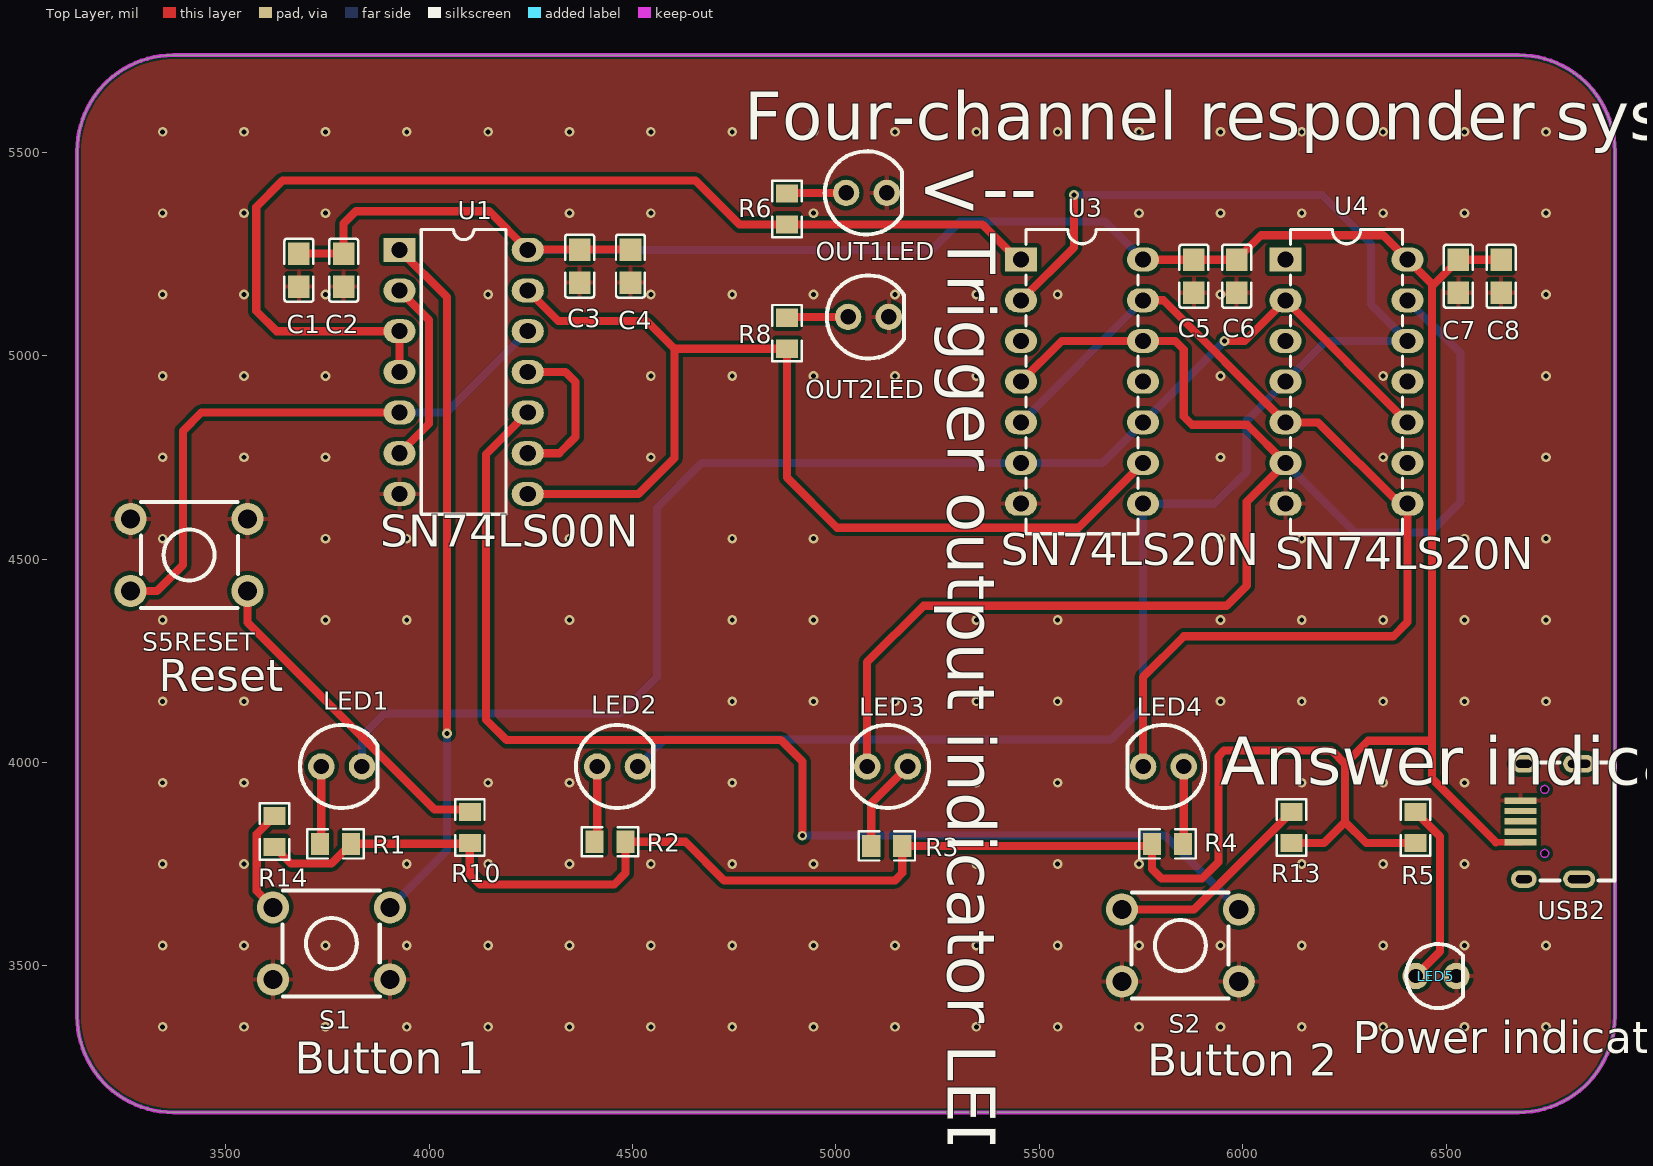
[diagram p0: Top Layer view]
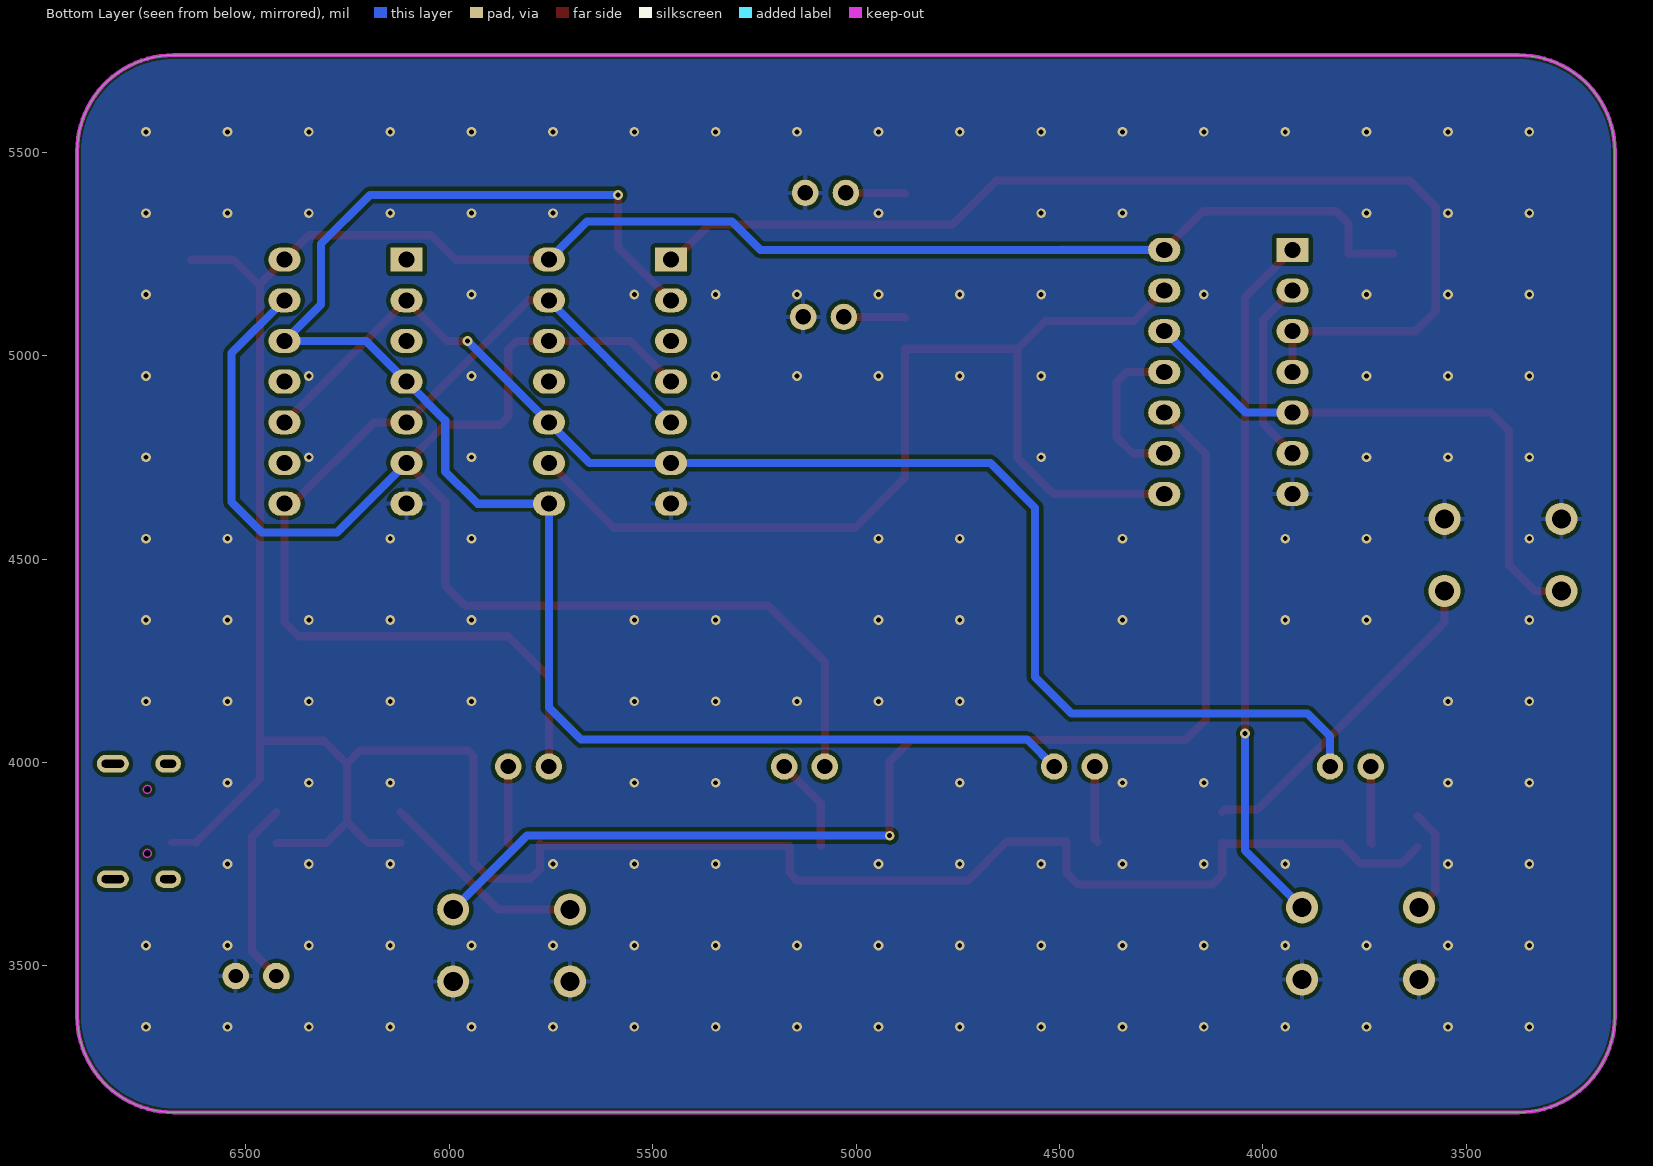
[diagram p1: Bottom Layer view, seen from below]
# Altium PCB MISC75096.pcbdoc
Units mil, origin at the board's own origin, x right, y up, seen from the top; angles counter-clockwise.
Board outline 3779.53 x 2598.43 mil, 2 copper layers (Top Layer, Bottom Layer), stack 62.206 mil thick; 32 components, 29 nets, 113 pads, 159 vias.

## Layer stack, top to bottom
Top Solder Mask Layer: solder mask 0.394, Dk 3.3
Top Layer: signal copper 1.379
Dielectric1: surface 59.449, FR4, Dk 4.5
Bottom Layer: signal copper 1.378
Bottom Solder Mask Layer: solder mask 0.394, Dk 3.3

## Board outline
3135,5502.2 cw(c3371.22,5502.2) 3371.22,5738.43 6678.31,5738.43 cw(c6678.31,5502.2) 6914.53,5502.2 6914.53,3376.22 cw(c6678.31,3376.22) 6678.31,3140 3371.22,3140 cw(c3371.22,3376.22) 3135,3376.22

## Design rules (kind name [scope] priority, off if disabled: settings)
BoardOutlineClearance Plane_innerPlane_1 [All] p2 off: genericclearance=6 ignorepadtopadclearanceinfootprint=FALSE except(0: Arc-SplitContinuation Track-SplitContinuation SMDPad-SplitContinuation THPad-SplitContinuation Via-SplitContinuation Fill-SplitContinuation Region-SplitContinuation Poly-SplitContinuation Text-SplitContinuation Hole-SplitContinuation; 6: Arc-CutoutEdge Track-CutoutEdge SMDPad-CutoutEdge THPad-CutoutEdge Via-CutoutEdge Fill-CutoutEdge Region-CutoutEdge Text-CutoutEdge; 6.9: Hole-OutlineEdge Hole-CutoutEdge; 10: Poly-OutlineEdge Poly-CutoutEdge; 11.8: Arc-OutlineEdge Track-OutlineEdge SMDPad-OutlineEdge THPad-OutlineEdge Via-OutlineEdge Fill-OutlineEdge Region-OutlineEdge Text-OutlineEdge)
BoardOutlineClearance Copper_copperRegion_1 [All] p4 off: genericclearance=6 ignorepadtopadclearanceinfootprint=FALSE except(0: Arc-SplitContinuation Track-SplitContinuation SMDPad-SplitContinuation THPad-SplitContinuation Via-SplitContinuation Fill-SplitContinuation Region-SplitContinuation Poly-SplitContinuation Text-SplitContinuation Hole-SplitContinuation; 6: Arc-CutoutEdge Track-CutoutEdge SMDPad-CutoutEdge THPad-CutoutEdge Via-CutoutEdge Fill-CutoutEdge Region-CutoutEdge Text-CutoutEdge; 6.9: Hole-OutlineEdge Hole-CutoutEdge; 10: Poly-OutlineEdge Poly-CutoutEdge; 11.8: Arc-OutlineEdge Track-OutlineEdge SMDPad-OutlineEdge THPad-OutlineEdge Via-OutlineEdge Fill-OutlineEdge Region-OutlineEdge Text-OutlineEdge)
BoardOutlineClearance Copper_gge8956_1 [All] p6 off: genericclearance=6 ignorepadtopadclearanceinfootprint=FALSE except(0: Arc-SplitContinuation Track-SplitContinuation SMDPad-SplitContinuation THPad-SplitContinuation Via-SplitContinuation Fill-SplitContinuation Region-SplitContinuation Poly-SplitContinuation Text-SplitContinuation Hole-SplitContinuation; 6: Arc-CutoutEdge Track-CutoutEdge SMDPad-CutoutEdge THPad-CutoutEdge Via-CutoutEdge Fill-CutoutEdge Region-CutoutEdge Text-CutoutEdge; 6.9: Hole-OutlineEdge Hole-CutoutEdge; 10: Poly-OutlineEdge Poly-CutoutEdge; 11.8: Arc-OutlineEdge Track-OutlineEdge SMDPad-OutlineEdge THPad-OutlineEdge Via-OutlineEdge Fill-OutlineEdge Region-OutlineEdge Text-OutlineEdge)
BoardOutlineClearance Copper_gge8950_1 [All] p8 off: genericclearance=6 ignorepadtopadclearanceinfootprint=FALSE except(0: Arc-SplitContinuation Track-SplitContinuation SMDPad-SplitContinuation THPad-SplitContinuation Via-SplitContinuation Fill-SplitContinuation Region-SplitContinuation Poly-SplitContinuation Text-SplitContinuation Hole-SplitContinuation; 6: Arc-CutoutEdge Track-CutoutEdge SMDPad-CutoutEdge THPad-CutoutEdge Via-CutoutEdge Fill-CutoutEdge Region-CutoutEdge Text-CutoutEdge; 6.9: Hole-OutlineEdge Hole-CutoutEdge; 10: Poly-OutlineEdge Poly-CutoutEdge; 11.8: Arc-OutlineEdge Track-OutlineEdge SMDPad-OutlineEdge THPad-OutlineEdge Via-OutlineEdge Fill-OutlineEdge Region-OutlineEdge Text-OutlineEdge)
BoardOutlineClearance safeClearance_1 [All] p10: genericclearance=6 ignorepadtopadclearanceinfootprint=FALSE except(0: Arc-SplitContinuation Track-SplitContinuation SMDPad-SplitContinuation THPad-SplitContinuation Via-SplitContinuation Fill-SplitContinuation Region-SplitContinuation Poly-SplitContinuation Text-SplitContinuation Hole-SplitContinuation; 6: Arc-CutoutEdge Track-CutoutEdge SMDPad-CutoutEdge THPad-CutoutEdge Via-CutoutEdge Fill-CutoutEdge Region-CutoutEdge Text-CutoutEdge; 6.9: Hole-OutlineEdge Hole-CutoutEdge; 10: Poly-OutlineEdge Poly-CutoutEdge; 11.8: Arc-OutlineEdge Track-OutlineEdge SMDPad-OutlineEdge THPad-OutlineEdge Via-OutlineEdge Fill-OutlineEdge Region-OutlineEdge Text-OutlineEdge)
Clearance Plane_innerPlane [All] p1 off: gap=6 ignorepadtopadclearanceinfootprint=FALSE except(6.9: Hole-Track Hole-SMDPad Hole-THPad Hole-Via Fill-Hole Region-Hole Hole-Arc Hole-Text; 10: Poly-Track Poly-SMDPad Poly-THPad Poly-Via Poly-Fill Poly-Region Poly-Poly Poly-Arc Poly-Text Poly-Hole)
Clearance Copper_copperRegion [All] p3 off: gap=6 ignorepadtopadclearanceinfootprint=FALSE except(6.9: Hole-Track Hole-SMDPad Hole-THPad Hole-Via Fill-Hole Region-Hole Hole-Arc Hole-Text; 10: Poly-Track Poly-SMDPad Poly-THPad Poly-Via Poly-Fill Poly-Region Poly-Poly Poly-Arc Poly-Text Poly-Hole)
Clearance Copper_gge8956 [All] p5 off: gap=6 ignorepadtopadclearanceinfootprint=FALSE except(6.9: Hole-Track Hole-SMDPad Hole-THPad Hole-Via Fill-Hole Region-Hole Hole-Arc Hole-Text; 10: Poly-Track Poly-SMDPad Poly-THPad Poly-Via Poly-Fill Poly-Region Poly-Poly Poly-Arc Poly-Text Poly-Hole)
Clearance Copper_gge8950 [All] p7 off: gap=6 ignorepadtopadclearanceinfootprint=FALSE except(6.9: Hole-Track Hole-SMDPad Hole-THPad Hole-Via Fill-Hole Region-Hole Hole-Arc Hole-Text; 10: Poly-Track Poly-SMDPad Poly-THPad Poly-Via Poly-Fill Poly-Region Poly-Poly Poly-Arc Poly-Text Poly-Hole)
Clearance safeClearance [All] p9: gap=6 ignorepadtopadclearanceinfootprint=FALSE except(6.9: Hole-Track Hole-SMDPad Hole-THPad Hole-Via Fill-Hole Region-Hole Hole-Arc Hole-Text; 10: Poly-Track Poly-SMDPad Poly-THPad Poly-Via Poly-Fill Poly-Region Poly-Poly Poly-Arc Poly-Text Poly-Hole)
DiffPairsRouting differentialPair [All] p1: maxlimit=6 minlimit=6 mostfreqgap=6 toplayer_minwidth=5 toplayer_prefwidth=10 toplayer_maxwidth=100 toplayer_mingap=6 toplayer_prefgap=6 toplayer_maxgap=6 bottomlayer_minwidth=5 bottomlayer_prefwidth=10 bottomlayer_maxwidth=100 bottomlayer_mingap=6 bottomlayer_prefgap=6 bottomlayer_maxgap=6 maxuncoupledlength=10
HoleToHoleClearance gge8956 [All] p1 off: gap=0 allowstackedmicrovias=TRUE
HoleToHoleClearance gge8950 [All] p2 off: gap=0 allowstackedmicrovias=TRUE
HoleToHoleClearance Common [All] p3: gap=11.8 allowstackedmicrovias=TRUE
Length netLength [All] p1: minlimit=0 maxlimit=0
PasteMaskExpansion pasteMaskExpansion [All] p1: expansion=0
PlaneConnect innerPlane [All] p1: planeconnectstyle=Relief reliefexpansion=20 reliefentries=4 reliefconductorwidth=10 reliefairgap=10
PolygonConnect gge8956_1 [All] p1 off: connectstyle=Relief reliefconductorwidth=10 reliefentries=4 polygonreliefangle="90 Angle" airgapwidth=10 via.connectstyle=Relief via.reliefconductorwidth=10 via.reliefentries=4 via.polygonreliefangle="90 Angle" via.airgapwidth=10
PolygonConnect gge8950_1 [All] p2 off: connectstyle=Relief reliefconductorwidth=10 reliefentries=4 polygonreliefangle="90 Angle" airgapwidth=10 via.connectstyle=Relief via.reliefconductorwidth=10 via.reliefentries=4 via.polygonreliefangle="90 Angle" via.airgapwidth=10
PolygonConnect copperRegion [All] p3: connectstyle=Relief reliefconductorwidth=10 reliefentries=4 polygonreliefangle="90 Angle" airgapwidth=10 via.connectstyle=Relief via.reliefconductorwidth=10 via.reliefentries=4 via.polygonreliefangle="90 Angle" via.airgapwidth=10
RoutingVias viaSize [All] p1: holewidth=12 width=24 viastyle="Through Hole" minholewidth=11.8 minwidth=19.7 maxholewidth=236.2 maxwidth=393.7
SolderMaskExpansion solderMaskExpansion [IsVia] p1: expansion=-1000 istentingtop=TRUE
SolderMaskExpansion solderMaskExpansion [All] p2: expansion=2 istentingtop=FALSE
Width trackWidth [All] p1: maxlimit=100 minlimit=5 preferedwidth=20

## Components (designator, comment, footprint, x,y, rotation, side; value= is the part's Value field where it differs from the comment)
C1 "10u" C0805 3680,5210 r270 top
C2 "0.1u" C0805 3790,5210 r270 top
C3 "10u" C0805 4370,5220 r270 top
C4 "0.1u" C0805 4495,5220 r270 top
C5 "10u" C0805 5880,5195 r270 top
C6 "0.1u" C0805 5985,5195 r270 top
C7 "10u" C0805 6530,5195 r270 top
C8 "0.1u" C0805 6635,5195 r270 top
LED1 "LED-TH-5mm_R" LED-TH_BD5.0_RED 3785,3989.99 r90 top
LED2 "LED-TH-5mm_R" LED-TH_BD5.0_RED 4463.2,3989.99 r90 top
LED3 "LED-TH-5mm_R" LED-TH_BD5.0_RED 5126.8,3990 r270 top
LED4 "LED-TH-5mm_R" LED-TH_BD5.0_RED 5805,3990 r270 top
LED5 "LED-TH-3mm_R" LED-TH_BD3.0_RED 6475,3475 r90 top
OUT1LED "LED-TH-5mm_R" LED-TH_BD5.0_RED 5075,5400 r90 top
OUT2LED "LED-TH-5mm_R" LED-TH_BD5.0_RED 5080,5095 r90 top
R1 "1k" R0805 3770,3800 r0 top
R2 "1k" R0805 4445,3805 r0 top
R3 "1k" R0805 5125,3795 r0 top
R4 "1k" R0805 5815,3800 r180 top
R5 "1k" R0805 6425,3840 r90 top
R6 "1k" R0805 4880,5360 r90 top
R8 "1k" R0805 4880,5055 r90 top
R10 "1k" R0805 4100,3840 r90 top
R13 "1k" R0805 6120,3840 r90 top
R14 "1k" R0805 3620,3830 r90 top
S1 "TC-1157-B-A" KEY-TH_4P-L6.4-W6.0-P4.50-LS7.3-TL 3760,3555 r0 top
S2 "TC-1157-B-A" KEY-TH_4P-L6.4-W6.0-P4.50-LS7.3-TL 5846.67,3550 r0 top
S5RESET "TC-1157-B-A" KEY-TH_4P-L6.4-W6.0-P4.50-LS7.3-TL 3410,4510 r180 top
U1 "SN74LS00N" PDIP-14_L19.7-W6.6-P2.54-LS8.3-BL 4085,4960 r270 top
U3 "SN74LS20N" DIP-14_L19.0-W7.0-P2.54-LS7.6-BL 5605,4935.98 r270 top
U4 "SN74LS20N" DIP-14_L19.0-W7.0-P2.54-LS7.6-BL 6255,4935.98 r270 top
USB2 "U-F-M5DD-W-2-SUS" MICRO-USB-SMD_U-F-M5DD-W-2-SUS 6755,3855 r270 top

## Footprints (in the part's own frame and the unit in brackets; to place one, negate y for a bottom-side part, rotate by r counter-clockwise, add the part's x,y. Pads: shape width x height; smd on the part's side, far side on the other; paste and mask are expansions set on the pad)
C0805 [mm]
  rect 1.41x1.35 smd paste-100 mask+0.051: 1(-1.03,0) 2(1.03,0)
  silkscreen extent -1.96,-0.9 1.96,0.9
DIP-14_L19.0-W7.0-P2.54-LS7.6-BL [mm]
  rect 1.5x2 hole 1: 1(-7.62,-3.81)
  oval 1.5x2 hole 1: 2(-5.08,-3.81) 3(-2.54,-3.81) 4(0,-3.81) 5(2.54,-3.81) 6(5.08,-3.81) 7(7.62,-3.81) 8(7.62,3.81) 9(5.08,3.81) 10(2.54,3.81) 11(0,3.81) 12(-2.54,3.81) 13(-5.08,3.81) 14(-7.62,3.81)
  silkscreen extent -9.5,-3.5 9.5,3.5
KEY-TH_4P-L6.4-W6.0-P4.50-LS7.3-TL [mm]
  round 2 hole 1.2: 1(-3.65,2.25) 2(3.65,2.25) 3(-3.65,-2.25)
  round 2 hole 1.2 copper offset 0,0: 4(3.65,-2.25)
  silkscreen extent -3.05,-3.3 3.01,3.3
LED-TH_BD3.0_RED [mil]
  round 65 hole 35.43: 1(0,50) 2(0,-50)
  silkscreen extent -79,-66 79,73
LED-TH_BD5.0_RED [mil]
  round 65 hole 38: 1(0,50) 2(0,-50)
  silkscreen extent -102,-88 102,102
MICRO-USB-SMD_U-F-M5DD-W-2-SUS [mm]
  rect 0.4x2 smd paste-100 mask+0.051: 1(1.3,-1.825) 2(0.65,-1.825) 3(0,-1.825) 4(-0.65,-1.825) 5(-1.3,-1.825)
  oval 1.1x1.6 hole 0.5 slot 1 at 90 deg: 6(-3.6,-1.625) 8(3.6,-1.625)
  oval 1.1x2 hole 0.5 slot 1.4 at 90 deg: 7(-3.6,1.825) 9(3.6,1.825)
  Board Outline Layer circle w0.003: c-2,-0.325 r0.25
  Board Outline Layer circle w0.003: c2,-0.325 r0.25
  Board Outline Layer region: -2,-0.075 -1.892,-0.1 -1.805,-0.169 -1.756,-0.269 -1.756,-0.38 -1.805,-0.481 -1.892,-0.55 -2,-0.575 -2,-0.575 -2.108,-0.55 -2.195,-0.481 -2.244,-0.38 -2.244,-0.269 -2.195,-0.169 -2.108,-0.1 -2,-0.075
  Board Outline Layer region: -2,-0.075 -1.935,-0.083 -1.875,-0.108 -1.823,-0.148 -1.783,-0.2 -1.759,-0.26 -1.75,-0.325 -1.759,-0.39 -1.783,-0.45 -1.823,-0.502 -1.875,-0.541 -1.935,-0.566 -2,-0.575 -2.065,-0.566 -2.125,-0.541 -2.177,-0.502 -2.217,-0.45 -2.241,-0.39 -2.25,-0.325 -2.241,-0.26 -2.217,-0.2 -2.177,-0.148 -2.125,-0.108 -2.065,-0.083
  Board Outline Layer region: 2,-0.075 2.108,-0.1 2.195,-0.169 2.244,-0.269 2.244,-0.38 2.195,-0.481 2.108,-0.55 2,-0.575 2,-0.575 1.892,-0.55 1.805,-0.481 1.756,-0.38 1.756,-0.269 1.805,-0.169 1.892,-0.1 2,-0.075
  Board Outline Layer region: 2,-0.075 2.065,-0.083 2.125,-0.108 2.177,-0.148 2.217,-0.2 2.241,-0.26 2.25,-0.325 2.241,-0.39 2.217,-0.45 2.177,-0.502 2.125,-0.541 2.065,-0.566 2,-0.575 1.935,-0.566 1.875,-0.541 1.823,-0.502 1.783,-0.45 1.759,-0.39 1.75,-0.325 1.759,-0.26 1.783,-0.2 1.823,-0.148 1.875,-0.108 1.935,-0.083
  Multi-Layer board cut-out: -2,-0.075 -1.892,-0.1 -1.805,-0.169 -1.756,-0.269 -1.756,-0.38 -1.805,-0.481 -1.892,-0.55 -2,-0.575 -2,-0.575 -2.108,-0.55 -2.195,-0.481 -2.244,-0.38 -2.244,-0.269 -2.195,-0.169 -2.108,-0.1 -2,-0.075
  Multi-Layer board cut-out: 2,-0.075 2.108,-0.1 2.195,-0.169 2.244,-0.269 2.244,-0.38 2.195,-0.481 2.108,-0.55 2,-0.575 2,-0.575 1.892,-0.55 1.805,-0.481 1.756,-0.38 1.756,-0.269 1.805,-0.169 1.892,-0.1 2,-0.075
  silkscreen extent -3.68,-0.6 3.68,4.04
PDIP-14_L19.7-W6.6-P2.54-LS8.3-BL [mm]
  rect 1.5x2 hole 1: 1(-7.62,-4)
  oval 1.5x2 hole 1: 2(-5.08,-4) 3(-2.54,-4) 4(0,-4) 5(2.54,-4) 6(5.08,-4) 7(7.62,-4) 8(7.62,4) 9(5.08,4) 10(2.54,4) 11(0,4) 12(-2.54,4) 13(-5.08,4) 14(-7.62,4)
  silkscreen extent -8.89,-2.65 8.89,2.65
R0805 [mil]
  rect 44.59x54.21 smd paste-3937.01 mask+2: 1(-38.04,0) 2(38.04,0)
  silkscreen extent -69,-36 69,36

## Via types
v1: diameter 24, hole 12, Top Layer to Bottom Layer, 159 vias

## Nets (pads, with @x,y where several pads share a name; then routed paths per layer and width w, separated by ;. In a path a pad name is that pad's centre, name@x,y a point inside that pad or via, vN(x,y) a via of type N, cw(c..) or ccw(c..) an arc to the next point about the centre after c; other vN are vias at no path point)
$1N3: LED1.1 R1.1 | length 191.3
  Top Layer w20: R1.1 3735,3803.04 LED1.1
$1N4: LED2.1 R2.1 | length 187.6
  Top Layer w20: R2.1 4413.2,3811.24 LED2.1
$1N5: LED3.1 R3.1 | length 232.2
  Top Layer w20: R3.1 5086.96,3900.16 LED3.1
$1N6: LED4.1 R4.1 | length 190.8
  Top Layer w20: R4.1 5855,3801.96 LED4.1
$1N15: U3.11
$1N29: U4.11
$1N34: U3.3
$1N40: U4.3
$1N42: U1.9 U1.11 | length 397
  Top Layer w20: U1.9 4320,4760 4360,4800 4360,4935 4335,4960 U1.11
$1N45: U1.2 U1.6 | length 460
  Top Layer w20: U1.6 4000,4832.48 4000,5087.52 U1.2
$1N65: LED5.1 R5.2 | length 452.7
  Top Layer w20: LED5.1 6485,3535 6485,3818.04 R5.2
$1N68: OUT1LED.1 R6.2 | length 145.8
  Top Layer w20: R6.2 4881.96,5400 OUT1LED.1
$1N72: OUT2LED.1 R8.2 | length 150.8
  Top Layer w20: R8.2 4881.96,5095 OUT2LED.1
$1N80: R10.2 S5RESET.1 | length 816.5
  Top Layer w20: S5RESET.1 3553.7,4344.34 4013.7,3884.34 4093.7,3884.34 R10.2
$1N88: R13.2 S2.1 | length 516.2
  Top Layer w20: S2.1 5880.54,3638.58 R13.2
$1N89: R14.2 S1.1 | length 259.1
  Top Layer w20: S1.1 3576.3,3683.58 3576.3,3824.34 R14.2
GND: C1.2 C2.2 C3.2 C4.2 C5.2 C6.2 C7.2 C8.2 LED5.2 OUT1LED.2 OUT2LED.2 S1.3 S1.4 S2.3 S2.4 S5RESET.3 S5RESET.4 U1.7 U3.7 U4.7 USB2.5
  other v1: 3345.1,3350.1 3545.1,3350.1 3745.1,3350.1 3945.1,3350.1 4145.1,3350.1 4345.1,3350.1 4545.1,3350.1 4745.1,3350.1 4945.1,3350.1 5145.1,3350.1 5345.1,3350.1 5545.1,3350.1 5745.1,3350.1 5945.1,3350.1 6145.1,3350.1 6345.1,3350.1 6545.1,3350.1 6745.1,3350.1 3345.1,3550.1 3545.1,3550.1 3745.1,3550.1 3945.1,3550.1 4145.1,3550.1 4345.1,3550.1 4545.1,3550.1 4745.1,3550.1 4945.1,3550.1 5145.1,3550.1 5345.1,3550.1 5545.1,3550.1 5745.1,3550.1 5945.1,3550.1 6145.1,3550.1 6345.1,3550.1 6545.1,3550.1 6745.1,3550.1 3345.1,3750.1 3545.1,3750.1 3945.1,3750.1 4145.1,3750.1 4345.1,3750.1 4545.1,3750.1 4745.1,3750.1 4945.1,3750.1 5345.1,3750.1 5545.1,3750.1 5745.1,3750.1 6145.1,3750.1 6345.1,3750.1 6545.1,3750.1 3345.1,3950.1 3545.1,3950.1 4145.1,3950.1 4345.1,3950.1 4745.1,3950.1 5345.1,3950.1 5545.1,3950.1 6145.1,3950.1 6345.1,3950.1 6545.1,3950.1 3345.1,4150.1 3545.1,4150.1 4745.1,4150.1 4945.1,4150.1 5145.1,4150.1 5345.1,4150.1 5545.1,4150.1 5945.1,4150.1 6145.1,4150.1 6345.1,4150.1 6545.1,4150.1 6745.1,4150.1 3345.1,4350.1 3745.1,4350.1 3945.1,4350.1 4345.1,4350.1 4745.1,4350.1 4945.1,4350.1 5345.1,4350.1 5545.1,4350.1 5945.1,4350.1 6145.1,4350.1 6345.1,4350.1 6545.1,4350.1 6745.1,4350.1 3345.1,4550.1 3745.1,4550.1 3945.1,4550.1 4345.1,4550.1 4745.1,4550.1 4945.1,4550.1 5945.1,4550.1 6145.1,4550.1 6545.1,4550.1 6745.1,4550.1 3345.1,4750.1 3545.1,4750.1 3745.1,4750.1 4545.1,4750.1 5945.1,4750.1 6345.1,4750.1 6745.1,4750.1 3345.1,4950.1 3545.1,4950.1 3745.1,4950.1 4545.1,4950.1 4745.1,4950.1 4945.1,4950.1 5145.1,4950.1 5345.1,4950.1 5945.1,4950.1 6345.1,4950.1 6745.1,4950.1 3345.1,5150.1 3545.1,5150.1 3745.1,5150.1 4145.1,5150.1 4545.1,5150.1 4745.1,5150.1 4945.1,5150.1 5145.1,5150.1 5345.1,5150.1 5545.1,5150.1 5945.1,5150.1 6745.1,5150.1 3345.1,5350.1 3545.1,5350.1 3745.1,5350.1 4345.1,5350.1 4545.1,5350.1 4945.1,5350.1 5745.1,5350.1 5945.1,5350.1 6145.1,5350.1 6345.1,5350.1 6545.1,5350.1 6745.1,5350.1 3345.1,5550.1 3545.1,5550.1 3745.1,5550.1 3945.1,5550.1 4145.1,5550.1 4345.1,5550.1 4545.1,5550.1 4745.1,5550.1 4945.1,5550.1 5145.1,5550.1 5345.1,5550.1 5545.1,5550.1 5745.1,5550.1 5945.1,5550.1 6145.1,5550.1 6345.1,5550.1 6545.1,5550.1 6745.1,5550.1
O1: R6.1 U1.3 U1.4 U3.1 | length 2715.5
  Top Layer w20: U1.4 U1.3 3625,5060 3575,5110 3575,5365 3640,5430 4655,5430 4763.04,5321.96 R6.1 5360,5321.96 5445.98,5235.98 U3.1
O2: R8.1 U1.8 U1.13 U3.9 | length 2671.5
  Top Layer w20: U1.8 4515,4660 4603.04,4748.04 4603.04,5016.96 ; U1.13 4317.48,5085 4535,5085 4603.04,5016.96 ; U3.9 5595.98,4576.96 5003.04,4576.96 4880,4700 R8.1 4603.04,5016.96
O3: U4.1
O4: U4.9
R: S5RESET.2 U1.5 U1.12 | length 1434
  Top Layer w20: S5RESET.2 3331.42,4421.42 3395,4485 3395,4815 3440,4860 U1.5
  Bottom Layer w20: U1.5 4042.48,4860 U1.12
S1: S1.2 U1.1 | length 1722.5
  Top Layer w20: U1.1 4043.7,5143.82 v1(4043.7,4071.18)
  Bottom Layer w20: S1.2 4043.7,3783.58 v1(4043.7,4071.18)
S2: S2.2 U1.10 | length 2947.9
  Top Layer w20: U1.10 4140,4757.52 4140,4105 4190,4055 4865,4055 4917.48,4002.52 v1(4917.48,3820)
  Bottom Layer w20: v1(4917.48,3820) 5808.95,3820 S2.2
VCC: C1.1 C2.1 C3.1 C4.1 C5.1 C6.1 C7.1 C8.1 R1.2 R2.2 R3.2 R4.2 R5.1 R10.1 R13.1 R14.1 U1.14 U3.14 U4.14 USB2.1 | length 9057.7
  Top Layer w15.75: 6622.06,3803.82 USB2.1
  Top Layer w20: R14.1 3660,3751.96 3760,3751.96 R1.2 4098.04,3800 R10.1 4100,3725 4125,3700 4455,3700 4483.04,3728.04 R2.2 4630,3805 4725,3710 5145,3710 5163.04,3728.04 R3.2 5771.96,3795 R4.2@5776.96,3790 ; C1.1 C2.1 3790,5325 3820,5355 4147.48,5355 U1.14 4243.03,5260.55 C3.1 C4.1 ; U3.14 5755.43,5235.55 C5.1 C6.1 6045.43,5295.98 6345,5295.98 U4.14 6465,5175.98 6465,5170.55 ; R4.2 R4.2@5776.96,3790 ; R13.1 6199.56,3801.96 6251.52,3853.92 ; R5.1 6303.48,3801.96 6251.52,3853.92 ; 6622.06,3803.82 6465,3960.88 6465,4053.24 ; C8.1 C7.1 6465,5170.55 ; R4.2@5776.96,3790 5776.96,3738.04 5800,3715 5900,3715 5940,3755 5940,4015 5954.14,4029.14 6218.91,4029.14 6251.52,3996.52 ; 6251.52,3853.92 6251.52,3996.52 ; 6251.52,3996.52 6308.24,4053.24 6465,4053.24 ; 6465,4053.24 6465,5170.55
  Bottom Layer w20: U1.14 5235,5260 5305,5330 5660.98,5330 U3.14
Y1: LED1.2 U3.6 U3.10 U4.2 U4.10 | length 3456.6
  Top Layer w20: v1(5955,5035.98) 6005,5035.98 U4.2 U4.10
  Bottom Layer w20: LED1.2 3835,4065 3890,4120 4470,4120 4560,4210 4560,4625.98 4670,4735.98 U3.6 5655,4735.98 U3.10 v1(5955,5035.98)
Y2: LED2.2 U3.2 U3.8 U4.4 U4.12 | length 4061.2
  Top Layer w20: U3.2 5585,5265.98 v1(5585,5395)
  Bottom Layer w20: LED2.2 4579.19,4055.98 5675.98,4055.98 5755,4135 U3.8 5930.98,4635.98 6010,4715 6010,4840.98 U4.4 6205,5035.98 U4.12 6315,5125.98 6315,5275 6195,5395 v1(5585,5395)
Y3: LED3.2 U3.4 U3.12 U4.6 U4.13 | length 3602.3
  Top Layer w20: LED3.2 5076.8,4246.8 5215,4385 5960,4385 6010,4435 6010,4640.98 U4.6 6010.98,4830 5875,4830 5855,4850 5855,5015 5834.02,5035.98 U3.12 5555,5035.98 U3.4
  Bottom Layer w20: U4.6 6275.98,4565 6460,4565 6535,4640 6535,5005.98 U4.13
Y4: LED4.2 U3.5 U3.13 U4.5 U4.8 | length 2498.3
  Top Layer w20: LED4.2 5755,4210 5855,4310 6370,4310 6405,4345 U4.8 6385,4635.98 6185,4835.98 U4.5 5805,5135.98 U3.13
  Bottom Layer w20: U3.5 U3.13
pads on no net: USB2.2 USB2.3 USB2.4 USB2.6 USB2.7 USB2.8 USB2.9

## Polygon pours and split planes (outlines as drawn)
GND on Bottom Layer (solid, remove dead copper, pour order 2): 3000,6040 7050,6040 7050,3010 3030,3010 3030,3000
GND on Top Layer (solid, remove dead copper, pour order 0): 3045,5970 7040,5970 7040,3015 3055,3015 3055,3025

## Keep-outs
Board Outline Layer:
  the board outline again, w10

## Silkscreen, mask and mechanical layers (free items; w line width, h text height)
Top Silkscreen Layer:
  text "Four-channel responder system" at 4775,5530 h118.11
  text "<--" at 5200,5345 h137.79
  text "Trigger output indicator LED" at 5275,5300 h118.11 r270
  text "SN74LS00N" at 3880,4530 h78.74
  text "SN74LS20N" at 5405,4485 h78.74
  text "SN74LS20N" at 6080,4475 h78.74
  text "Reset" at 3335,4175 h78.74
  text "Answer indicator LED" at 5945,3945 h118.11
  text "Power indicator LED" at 6270,3285 h78.74
  text "Button 1" at 3670,3235 h78.74
  text "Button 2" at 5765,3230 h78.74
Top Solder Mask Layer:
  text "<--" at 5200,5345 h137.79
  text "Trigger output indicator LED" at 5275,5300 h118.11 r270
  text "Answer indicator LED" at 5945,3945 h118.11